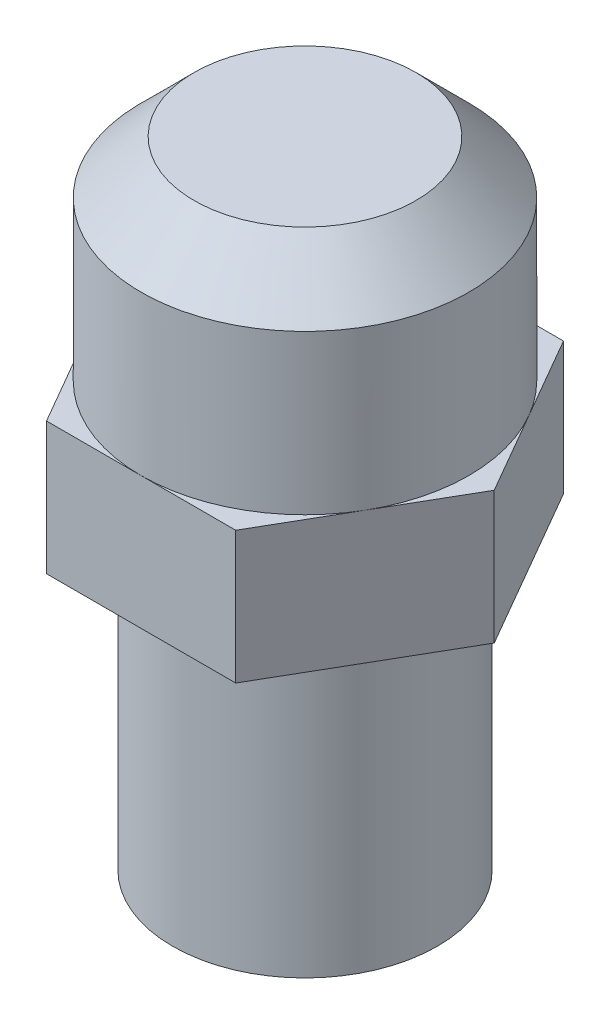
from build123d import *

# Parameters (mm, degrees)
EXTRUDE_1_DEPTH = 5
SKETCH_2_R      = 6.192081637
EXTRUDE_2_DEPTH = 8
CHAMFER_1_SIZE  = 2
SKETCH_3_R      = 5
EXTRUDE_3_DEPTH = 11


with BuildPart() as part:
    # 草图1 → 凸台-拉伸1 (new body)
    with BuildSketch(Plane(origin=(0, 0, 0), x_dir=(1, 0, 0), z_dir=(0, 1, 0))):
        Polygon((-7.15, 0), (-3.575, -6.192081637), (3.575, -6.192081637), (7.15, 0), (3.575, 6.192081637), (-3.575, 6.192081637), align=None)
    extrude(amount=EXTRUDE_1_DEPTH)

    # 草图2 → 凸台-拉伸2 (add)
    with BuildSketch(Plane(origin=(0, 5, 0), x_dir=(1, 0, 0), z_dir=(0, 1, 0))):
        with Locations(Location((0, 0, 0), (0, 0, 270))):
            Circle(SKETCH_2_R)
    extrude(amount=EXTRUDE_2_DEPTH)

    # 倒角1
    chamfer_1_edges = [part.edges().sort_by_distance(p)[0] for p in [
        (0, 13, -6.192081637),
    ]]
    chamfer(chamfer_1_edges, length=CHAMFER_1_SIZE)

    # 草图3 → 凸台-拉伸3 (add)
    with BuildSketch(Plane.XZ):
        with Locations(Location((0, 0, 0), (0, 0, 90))):
            Circle(SKETCH_3_R)
    extrude(amount=EXTRUDE_3_DEPTH)


solid = part.part
